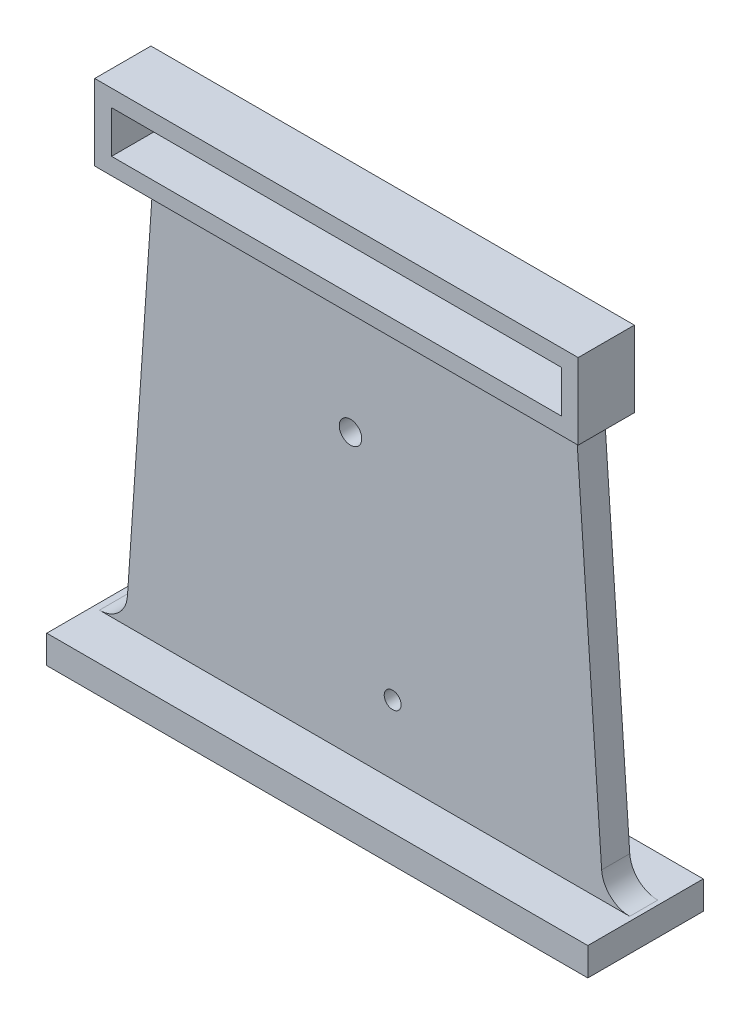
SolidWorks part; units mm, degrees
ref_plane "Front Plane" through (0, 0, 0) normal (0, 0, 1) x (1, 0, 0)
ref_plane "Top Plane" through (0, 0, 0) normal (0, 1, 0) x (1, 0, 0)
ref_plane "Right Plane" through (0, 0, 0) normal (1, 0, 0) x (0, 0, -1)
sketch "Sketch1" plane through (0, 0, 0) normal (0, 0, 1) x (1, 0, 0)
  line L0 (0, 0) -> (170, 0)
  line L1 (170, 0) -> (160, 146)
  line L2 (160, 146) -> (10, 146)
  line L3 (10, 146) -> (0, 0)
  line L4 (85, 0) -> (85, 181.1071) construction
  circle A0 centre (95, 24.5) radius 3
  circle A1 centre (80, 99.5) radius 4
  dimension "D5" = 6
  dimension "D6" = 8
  dimension "D7" = 46.5
  dimension "D9" = 10
  dimension "D10" = 75
  dimension "D1" = 170
  dimension "D2" = 150
  dimension "D3" = 10
  dimension "D4" = 146
  dimension "D8" = 85
  dimension "D11" = 5
extrude "Boss-Extrude1" add sketch "Sketch1" along normal blind 10
sketch "Sketch2" plane through (0, 0, 0) normal (0, -1, 0) x (-1, 0, 0)
  line L1 (11.6149, -26.4546) -> (-180.8915, -26.4546)
  line L2 (11.6149, -26.4546) -> (11.6149, 14.6175)
  line L3 (11.6149, 14.6175) -> (-180.8915, 14.6175)
  line L4 (-180.8915, -26.4546) -> (-180.8915, 14.6175)
  line L5 (11.6149, -26.4546) -> (-180.8915, 14.6175) construction
  line L6 (11.6149, 14.6175) -> (-180.8915, -26.4546) construction
  point P0 (-84.6383, -5.9186)
extrude "Boss-Extrude2" add sketch "Sketch2" along normal blind 10
fillet "Fillet1" radius 10 2 edges at (170, 0, 5) (0, 0, 5)
sketch "Sketch3" plane through (0, 0, 10) normal (0, 0, 1) x (1, 0, 0)
  line L0 (160, 146) -> (10, 146) construction
  line L1 (5, 152) -> (165, 152)
  line L2 (5, 152) -> (5, 167)
  line L3 (5, 167) -> (165, 167)
  line L4 (165, 152) -> (165, 167)
  line L5 (-1, 173) -> (171, 173)
  line L6 (-1, 173) -> (-1, 146)
  line L7 (-1, 146) -> (171, 146)
  line L8 (171, 173) -> (171, 146)
  dimension "D1" = 15
  dimension "D2" = 160
  dimension "D3" = 5
  dimension "D4" = 6
  dimension "D5" = 6
  dimension "D6" = 6
  dimension "D7" = 6
  dimension "D8" = 0
extrude "Boss-Extrude3" add sketch "Sketch3" against normal mid plane 20
